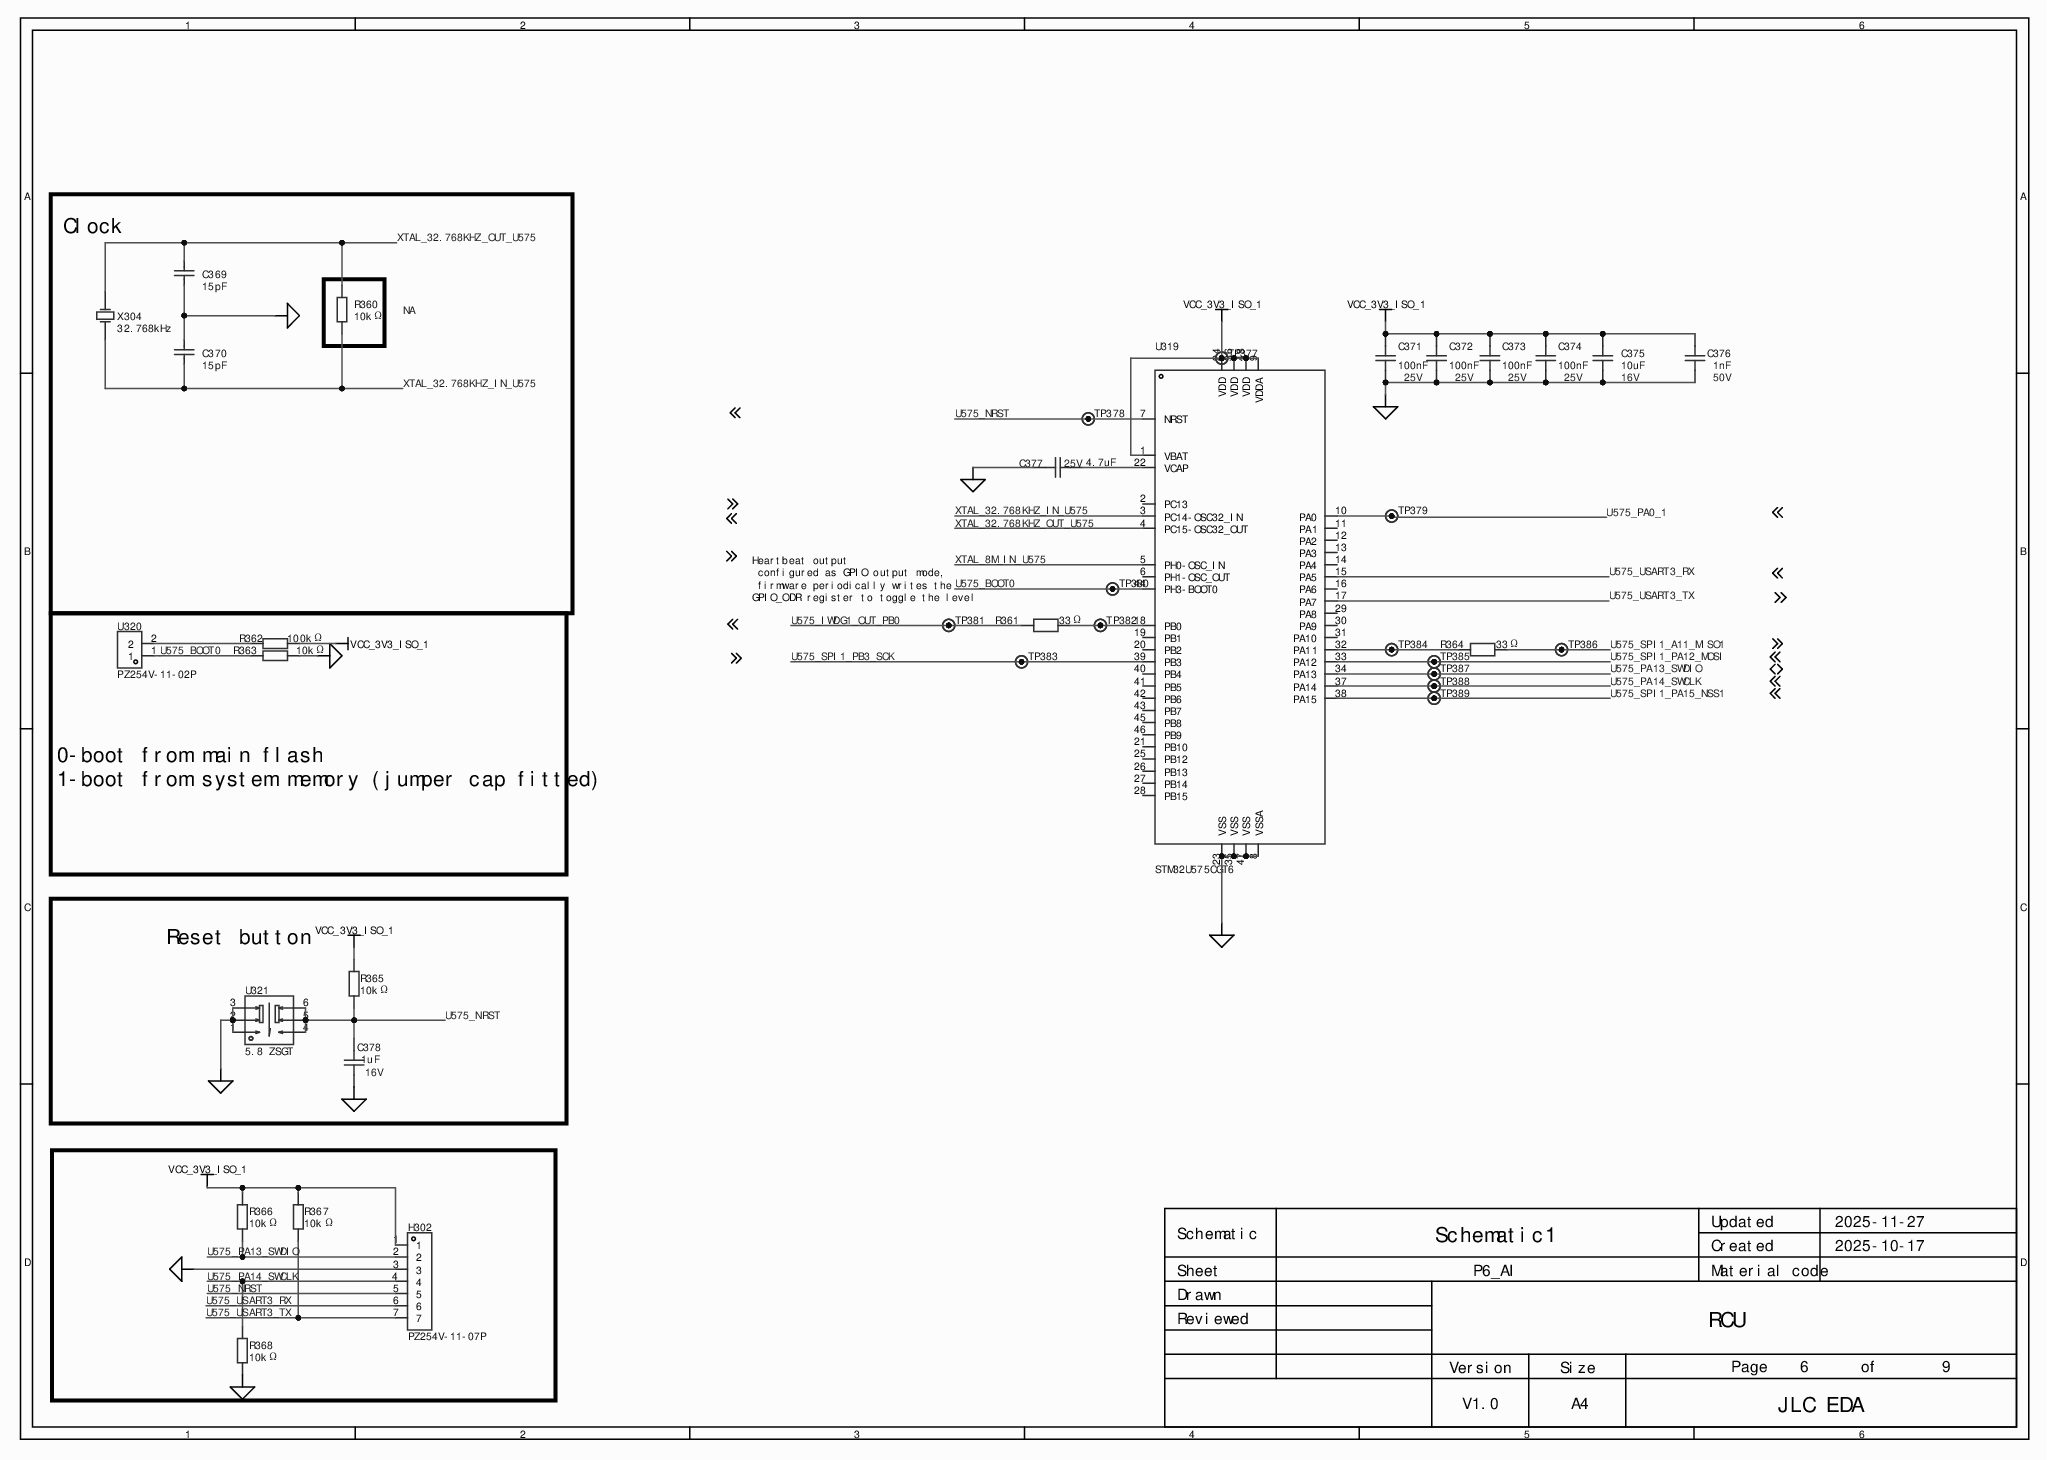
[diagram p0: MISC84429-7.SchDoc]
# Altium project MISC84429-12.PrjPcb (part 1 of 5)
9 sheets, 424 parts. Net scope: global (net labels, ports and power ports of the same name join across sheets).
Board file: MISC84429.PcbDoc
Sheets:
  MISC84429-7.SchDoc
  MISC84429-4.SchDoc
  MISC84429-3.SchDoc
  MISC84429-2.SchDoc
  MISC84429-5.SchDoc
  MISC84429-6.SchDoc
  MISC84429-8.SchDoc
  MISC84429-10.SchDoc
  MISC84429-9.SchDoc

## Sheet MISC84429-7.SchDoc
size 431 x 309 mm; Name: Sheet-Symbol; Symbol: Sheet-Symbol; Device: Sheet-Symbol

### Parts
C369  15pF  [C0402]
C370  15pF  [C0402]
C371  100nF  Voltage Rated: 25V  [C0603]
C372  100nF  Voltage Rated: 25V  [C0603]
C373  100nF  Voltage Rated: 25V  [C0603]
C374  100nF  Voltage Rated: 25V  [C0603]
C375  10uF  Voltage Rated: 16V  [C0805]
C376  1nF  Voltage Rated: 50V  [C0603]
C377  4.7uF  Voltage Rating: 25V  [C0603]
C378  1uF  Voltage Rated: 16V  [C0603]
H302  PZ254V-11-07P  [HDR-TH_7P-P2.54-V-M]
R360  10kΩ  [R0402]
R361  33Ω  [R0603]
R362  100kΩ  [R0603]
R363  10kΩ  [R0603]
R364  33Ω  [R0603]
R365  10kΩ  [R0603]
R366  10kΩ  [R0603]
R367  10kΩ  [R0603]
R368  10kΩ  [R0603]
TP377  (no value)  [Test-Point-0.5mm]
TP378  (no value)  [Test-Point-0.5mm]
TP379  (no value)  [Test-Point-0.5mm]
TP380  (no value)  [Test-Point-0.5mm]
TP381  (no value)  [Test-Point-0.5mm]
TP382  (no value)  [Test-Point-0.5mm]
TP383  (no value)  [Test-Point-0.5mm]
TP384  (no value)  [Test-Point-0.5mm]
TP385  (no value)  [Test-Point-0.5mm]
TP386  (no value)  [Test-Point-0.5mm]
TP387  (no value)  [Test-Point-0.5mm]
TP388  (no value)  [Test-Point-0.5mm]
TP389  (no value)  [Test-Point-0.5mm]
U319  STM32U575CGT6  [LQFP-48_L7.0-W7.0-P0.50-LS9.0-TL]
U320  PZ254V-11-02P  [HDR-TH_2P-P2.54-V-M]
U321  5.8 ZSGT  [SW-TH_5.8ZSGT]
X304  32.768kHz  [OSC-TH_BD3.1-P0.8-D0.3]

### Blocks framed on the sheet
Clock: C369 C370 R360 X304
Reset button: C378 R365 U321

### Nets
PGND: C369.1 C370.2 C371.2 C372.2 C373.2 C374.2 C375.1 C376.1 C377.2 C378.1 H302.3 R363.2 R368.2 U319.8(VSSA) U319.23(VSS) U319.35(VSS) U319.47(VSS) U321.1 U321.2 U321.3
VCC_3V3_ISO_1: C371.1 C372.1 C373.1 C374.1 C375.2 C376.2 H302.1 R362.2 R365.2 R366.2 R367.2 TP377.1 U319.1(VBAT) U319.9(VDDA) U319.24(VDD) U319.36(VDD) U319.48(VDD)
U575_BOOT0: R363.1 TP380.1 U319.44(PH3-BOOT0) U320.1
U575_IWDG1_OUT_PB0: R361.2 TP381.1
U575_NRST: C378.2 H302.5 R365.1 TP378.1 U319.7(NRST) U321.4 U321.5 U321.6
U575_PA0_1: TP379.1 U319.10(PA0)
U575_PA13_SWDIO: H302.2 R366.1 TP387.1 U319.34(PA13)
U575_PA14_SWCLK: H302.4 R368.1 TP388.1 U319.37(PA14)
U575_SPI1_A11_MISO1: R364.1 TP386.1
U575_SPI1_PA12_MOSI: TP385.1 U319.33(PA12)
U575_SPI1_PA15_NSS1: TP389.1 U319.38(PA15)
U575_SPI1_PB3_SCK: TP383.1 U319.39(PB3)
U575_USART3_RX: H302.6 U319.15(PA5)
U575_USART3_TX: H302.7 R367.1 U319.17(PA7)
XTAL_8M_IN_U575: U319.5(PH0-OSC_IN)
XTAL_32.768KHZ_IN_U575: C370.1 R360.1 U319.3(PC14-OSC32_IN) X304.1(OSC1)
XTAL_32.768KHZ_OUT_U575: C369.2 R360.2 U319.4(PC15-OSC32_OUT) X304.2(OSC2)
NetC377_1: C377.1 U319.22(VCAP)
NetR361_1: R361.1 TP382.1 U319.18(PB0)
NetR362_1: R362.1 U320.2
NetR364_2: R364.2 TP384.1 U319.32(PA11)

Not connected (* = marked no-connect by the designer): U319 2(PC13)* 6(PH1-OSC_OUT)* 11(PA1)* 12(PA2)* 13(PA3)* 14(PA4)* 16(PA6)* 19(PB1)* 20(PB2)* 21(PB10)* 25(PB12)* 26(PB13)* 27(PB14)* 28(PB15)* 29(PA8)* 30(PA9)* 31(PA10)* 40(PB4)* 41(PB5)* 42(PB6)* 43(PB7)* 45(PB8)* 46(PB9)*

### Notes on the sheet
- NA
- Heartbeat output
  configured as GPIO output mode,
  firmware periodically writes the
  GPIO_ODR register to toggle the level
- 0-boot from main flash
  1-boot from system memory (jumper cap fitted)
- 1
- 2
- 3
- 4
- 5
- 6
- A
- B
- C
- D
- Schematic
- Schematic1
- Created
- Updated
- 2025-11-27
- 2025-10-17
- Reviewed
- Drawn
- Sheet
- P6_AI
- Material code
- RCU
- Version
- Size
- Page
- of
- 9
- V1.0
- A4
- JLC EDA

### Library data of the parts
C369 C370 = GJM1555C1H150FB01D: Manufacturer: muRata(村田); Add into BOM: yes; Tolerance: ±1%; Voltage Rated: 50V; Temperature Coefficient: C0G; Symbol: GJM1555C1H150FB01D; Device: GJM1555C1H150FB01D; LCSC Part Name: 15pF ±1% 50V; Supplier Part: C441742; Manufacturer Part: GJM1555C1H150FB01D; Supplier Footprint: 0402; JLCPCB Part Class: Extended library; Datasheet: https://atta.szlcsc.com/upload/public/pdf/source/20200305/C490387_23319AE8C154DEB24C505E6C82A8106A.pdf; Supplier: LCSC; Convert to PCB: yes; Value: 15pF; Origin Footprint: C0402
C371-C374 = GRM188R71E104KA01D: Manufacturer: muRata(村田); Add into BOM: yes; Tolerance: ±10%; Temperature Coefficient: X7R; Symbol: GRM188R71E104KA01D; Device: GRM188R71E104KA01D; LCSC Part Name: 100nF ±10% 25V; Supplier Part: C77050; Manufacturer Part: GRM188R71E104KA01D; Supplier Footprint: 0603; JLCPCB Part Class: Extended library; Datasheet: https://atta.szlcsc.com/upload/public/pdf/source/20170622/1498103881034.pdf; Supplier: LCSC; Convert to PCB: yes; Value: 100nF; Origin Footprint: C0603
C375 = GRM21BR61C106KE15L: Manufacturer: muRata(村田); Add into BOM: yes; Tolerance: ±10%; Temperature Coefficient: X5R; Symbol: GRM21BR61C106KE15L; Device: GRM21BR61C106KE15L; LCSC Part Name: 10uF ±10% 16V; Supplier Part: C77075; Manufacturer Part: GRM21BR61C106KE15L; Supplier Footprint: 0805; JLCPCB Part Class: Extended library; Datasheet: https://atta.szlcsc.com/upload/public/pdf/source/20200305/C490387_23319AE8C154DEB24C505E6C82A8106A.pdf; Supplier: LCSC; Convert to PCB: yes; Value: 10uF; Origin Footprint: C0805
C376 = GRM1885C1H102JA01D: Manufacturer: muRata(村田); Add into BOM: yes; Tolerance: ±5%; Temperature Coefficient: C0G; Symbol: GRM1885C1H102JA01D; Device: GRM1885C1H102JA01D; LCSC Part Name: 1nF ±5% 50V; Supplier Part: C77026; Manufacturer Part: GRM1885C1H102JA01D; Supplier Footprint: 0603; JLCPCB Part Class: Extended library; Datasheet: https://atta.szlcsc.com/upload/public/pdf/source/20200305/C490387_23319AE8C154DEB24C505E6C82A8106A.pdf; Supplier: LCSC; Convert to PCB: yes; Value: 1nF; Origin Footprint: C0603
C377 = GRM188R61E475KE11D: Manufacturer: muRata(村田); Add into BOM: yes; Tolerance: ±10%; Temperature Coefficient: X5R; Symbol: GRM188R61E475KE11D; Device: GRM188R61E475KE11D; LCSC Part Name: 4.7uF ±10% 25V; Supplier Part: C90057; Manufacturer Part: GRM188R61E475KE11D; Supplier Footprint: 0603; JLCPCB Part Class: Extended library; Datasheet: https://item.szlcsc.com/datasheet/GRM188R61E475KE11D/91242.html; Supplier: LCSC; Convert to PCB: yes; Value: 4.7uF; Origin Footprint: C0603
C378 = GCM188R71C105KA64D: Manufacturer: muRata(村田); Add into BOM: yes; Tolerance: ±10%; Temperature Coefficient: X7R; Symbol: GCM188R71C105KA64D; Device: GCM188R71C105KA64D; LCSC Part Name: 1uF ±10% 16V; Supplier Part: C161212; Manufacturer Part: GCM188R71C105KA64D; Supplier Footprint: 0603; JLCPCB Part Class: Extended library; Datasheet: https://atta.szlcsc.com/upload/public/pdf/source/20181221/C161212_C96DD77354D5551432B3B7779E4D1948.pdf; Supplier: LCSC; Convert to PCB: yes; Value: 1uF; Origin Footprint: C0603
H302 = PZ254V-11-07P: Manufacturer: XFCN(兴飞); Add into BOM: yes; Pin Structure: 1x7P; Pitch: 2.54mm; Circluar Pins/Square Pins: Square pin; Symbol: PZ254V-11-07P; Device: PZ254V-11-07P; LCSC Part Name: 1x7P 间距:2.54mm 方针 直插; Supplier Part: C492406; Manufacturer Part: PZ254V-11-07P; Supplier Footprint: 插件,P=2.54mm; JLCPCB Part Class: Extended library; Datasheet: https://atta.szlcsc.com/upload/public/pdf/source/20200309/C492406_654C533EE691117E22DD9F76C114C2D9.pdf; Supplier: LCSC; Convert to PCB: yes; Row Spacing: -; Mounting Type: Through hole; Number of Rows: Single row; Number of Pins: 7P; Current Rating: -; Voltage Rating (Max): -; Length of Mating Pin: 6mm; Insulation Height: 2.5mm; Length of End Connection Pin: 3mm; Contact Material: Brass; Contact Plating: -; Operating Temperature: -40℃~+105℃; Color: Black; Origin Footprint: HDR-TH_7P-P2.54-V-M
R360 = 0402WGF1002TCE: Manufacturer: UNI-ROYAL(厚声); Add into BOM: yes; Tolerance: ±1%; Power(Watts): 62.5mW; Overload Voltage (Max): 50V; Temperature Coefficient: ±100ppm/℃; Symbol: 0402WGF1002TCE; Device: 0402WGF1002TCE; LCSC Part Name: 10kΩ ±1% 62.5mW 厚膜电阻; Supplier Part: C25744; Manufacturer Part: 0402WGF1002TCE; Supplier Footprint: 0402; JLCPCB Part Class: Basic library; Datasheet: https://atta.szlcsc.com/upload/public/pdf/source/20200306/C422600_1E6D84923E4A46A82E41ADD87F860B5C.pdf; Supplier: LCSC; Convert to PCB: yes; Type: Thick film resistor; Value: 10kΩ; Operating Temperature Range: -55℃~+155℃; Origin Footprint: R0402
R361 R364 = FRC0603F33R0TS: Manufacturer: FOJAN(富捷); Add into BOM: yes; Tolerance: ±1%; Power(Watts): 100mW; Voltage-Supply(Max): 75V; Temperature Coefficient: ±100ppm/℃; Symbol: FRC0603F33R0TS; Device: FRC0603F33R0TS; LCSC Part Name: 33Ω ±1% 100mW 厚膜电阻; Supplier Part: C2909394; Manufacturer Part: FRC0603F33R0TS; Supplier Footprint: 0603; JLCPCB Part Class: Extended library; Supplier: LCSC; Convert to PCB: yes; Type: Thick film resistor; Value: 33Ω; Operating Temperature: -55℃~+155℃; Origin Footprint: R0603
R362 = RC0603FR-07100KL: Manufacturer: YAGEO(国巨); Add into BOM: yes; Tolerance: ±1%; Power(Watts): 100mW; Overload Voltage (Max): 75V; Temperature Coefficient: ±100ppm/℃; Symbol: RC0603FR-07100KL; Device: RC0603FR-07100KL; LCSC Part Name: 厚膜电阻 100kΩ ±1% 100mW; Supplier Part: C14675; Manufacturer Part: RC0603FR-07100KL; Supplier Footprint: 0603; JLCPCB Part Class: Extended library; Datasheet: https://atta.szlcsc.com/upload/public/pdf/source/20140324/1457707028752.pdf; Supplier: LCSC; Convert to PCB: yes; Type: Thick film resistor; Value: 100kΩ; Operating Temperature Range: -55℃~+155℃; Origin Footprint: R0603
R363 R365-R368 = RC0603FR-0710KL: Manufacturer: YAGEO(国巨); Add into BOM: yes; Tolerance: ±1%; Power(Watts): 100mW; Overload Voltage (Max): 75V; Temperature Coefficient: ±100ppm/℃; Symbol: RC0603FR-0710KL; Device: RC0603FR-0710KL; LCSC Part Name: 厚膜电阻 10kΩ ±1% 100mW; Supplier Part: C98220; Manufacturer Part: RC0603FR-0710KL; Supplier Footprint: 0603; JLCPCB Part Class: Extended library; Datasheet: https://atta.szlcsc.com/upload/public/pdf/source/20180927/C295883_E8D83085EA81BD7DE0B2B681138C15EE.pdf; Supplier: LCSC; Convert to PCB: yes; Type: Thick film resistor; Value: 10kΩ; Operating Temperature Range: -55℃~+155℃; Origin Footprint: R0603
TP377-TP389 = Test-Point: Add into BOM: yes; Symbol: Test-Point; Device: Test-Point; Convert to PCB: yes; Origin Footprint: Test-Point-0.5mm
U319 = STM32U575CGT6: Manufacturer: ST(意法半导体); Add into BOM: yes; Symbol: STM32U575CGT6; Device: STM32U575CGT6; LCSC Part Name: 超低功耗带 FPU 的 Arm Cortex-M33 具有 Trust Zone，160 MHz MCU 带 1MB 闪存; Supplier Part: C5271006; Manufacturer Part: STM32U575CGT6; Supplier Footprint: LQFP-48(7x7); JLCPCB Part Class: Extended library; Datasheet: https://atta.szlcsc.com/upload/public/pdf/source/20250311/118E46867C2F8A0EF1AEA9206C957AC0.pdf; Supplier: LCSC; Convert to PCB: yes; Origin Footprint: LQFP-48_L7.0-W7.0-P0.50-LS9.0-TL
U320 = PZ254V-11-02P: Manufacturer: XFCN(兴飞); Add into BOM: yes; Pin Structure: 1x2P; Pitch: 2.54mm; Circluar Pins/Square Pins: Square pin; Symbol: PZ254V-11-02P; Device: PZ254V-11-02P; LCSC Part Name: 间距:2.54mm 1x2P 直插 方针; Supplier Part: C492401; Manufacturer Part: PZ254V-11-02P; Supplier Footprint: 插件,P=2.54mm; JLCPCB Part Class: Extended library; Datasheet: https://atta.szlcsc.com/upload/public/pdf/source/20200309/C492401_A812433581A9B211A7FFA413ADDFF0E5.pdf; Supplier: LCSC; Convert to PCB: yes; Row Spacing: -; Mounting Type: Through hole; Number of Rows: Single row; Number of Pins: 2P; Current Rating (Max): -; Voltage Rating (Max): -; Length of Mating Pin: 6mm; Insulation Height: 2.5mm; Length of End Connection Pin: 3mm; Contact Material: Brass; Contact Plating: -; Operating Temperature Range: -40℃~+105℃; Color: Black; Origin Footprint: HDR-TH_2P-P2.54-V-M
U321 = 5.8 ZSGT: Manufacturer: SHOU HAN(首韩); Add into BOM: yes; Circuit: DPDT; Self Lock / No Lock: Self-locking; Actuator Style: Square button; Contact Current: 110mA; Voltage Rating (DC): 30V; Insulation Resistance: 100MΩ; Actuator/Cap Color: White; With Lamp: Without; Pin Style: PC pin; Operating Force: 1.5N; Mechanical Life: 10 ten-thousand cycles; Symbol: 5.8 ZSGT; Device: 5.8 ZSGT; LCSC Part Name: 5.8*5.8有头/高头 带锁/自锁开关 泡泡机开关; Supplier Part: C2681587; Manufacturer Part: 5.8 ZSGT; Supplier Footprint: 插件; JLCPCB Part Class: Extended library; Datasheet: https://atta.szlcsc.com/upload/public/pdf/source/20210107/C2681587_CDDDDA4A1C7AC9FEB01815B75893A6BA.pdf; Supplier: LCSC; Convert to PCB: yes; Mounting Style: Through hole; Operating Temperature: -10℃~+70℃; Origin Footprint: SW-TH_5.8ZSGT
X304 = X308032768KGB2SC: Manufacturer: YXC(扬兴晶振); Add into BOM: yes; Normal temperature Frequency Tolerance: ±10ppm; Load Capacitance: 12.5pF; Frequency Stability: ±20ppm; Symbol: X308032768KGB2SC; Device: X308032768KGB2SC; LCSC Part Name: YT-38 32.768KHZ 2P 3080 12.5PF ±10PPM -20~70℃; Supplier Part: C52082; Manufacturer Part: X308032768KGB2SC; Supplier Footprint: DT-38; JLCPCB Part Class: Extended library; Datasheet: https://item.szlcsc.com/datasheet/X308032768KGB2SC/53096.html; Supplier: LCSC; Convert to PCB: yes; Type: Through-hole crystal; Value: 32.768kHz; Operating Temperature: -20℃~+70℃; Origin Footprint: OSC-TH_BD3.1-P0.8-D0.3

## Sheet MISC84429-4.SchDoc
size 431 x 309 mm; Name: Sheet-Symbol; Symbol: Sheet-Symbol; Device: Sheet-Symbol
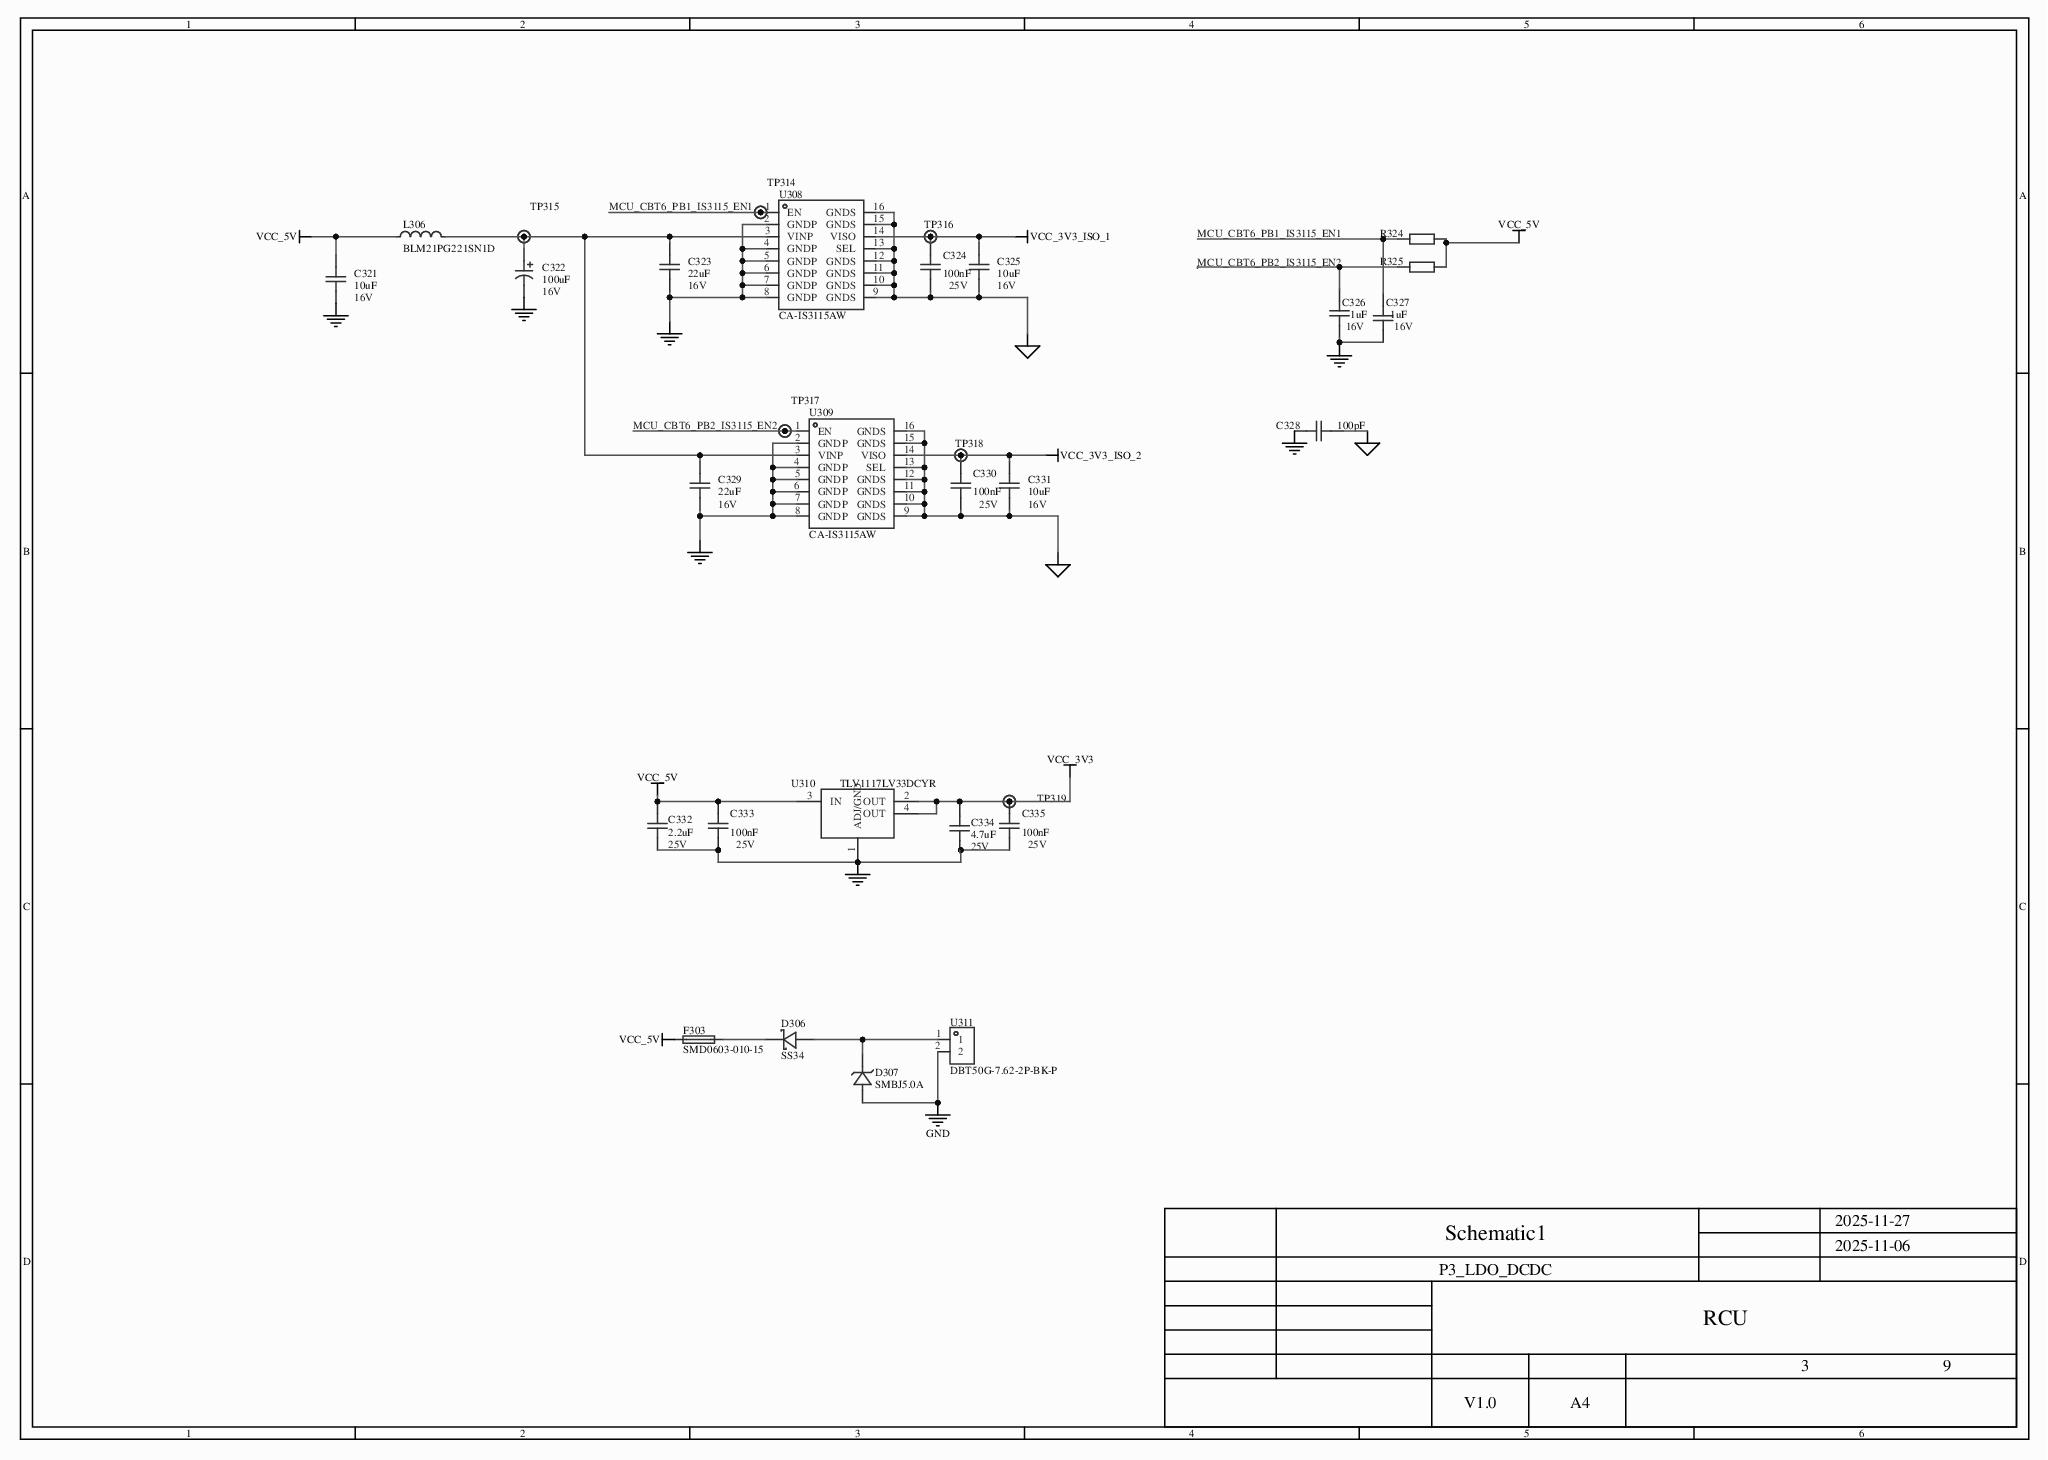
[diagram p1: MISC84429-4.SchDoc]

### Parts
C321  10uF  Voltage Rated: 16V  [C0805]
C322  100uF  Voltage Rating: 16V  [CAP-SMD_BD6.3-L6.6-W6.6-LS7.2-FD]
C323  22uF  Voltage Rating: 16V  [C0603]
C324  100nF  Voltage Rated: 25V  [C0603]
C325  10uF  Voltage Rated: 16V  [C0805]
C326  1uF  Voltage Rated: 16V  [C0603]
C327  1uF  Voltage Rated: 16V  [C0603]
C328  100pF  [CAP-TH_L7.0-W4.0-P10.00-D0.6]
C329  22uF  Voltage Rating: 16V  [C0603]
C330  100nF  Voltage Rated: 25V  [C0603]
C331  10uF  Voltage Rated: 16V  [C0805]
C332  2.2uF  Voltage Rating: 25V  [C0603]
C333  100nF  Voltage Rated: 25V  [C0603]
C334  4.7uF  Voltage Rating: 25V  [C0603]
C335  100nF  Voltage Rated: 25V  [C0603]
D306  SS34  [SMC_L6.9-W5.9-LS7.9-RD]
D307  SMBJ5.0A  [SMB_L4.6-W3.6-LS5.4-RD]
F303  SMD0603-010-15  [F0603]
L306  BLM21PG221SN1D  [L0805]
R324  (no value)  [R0603]
R325  (no value)  [R0603]
TP314  (no value)  [Test-Point-0.5mm]
TP315  (no value)  [Test-Point-0.5mm]
TP316  (no value)  [Test-Point-0.5mm]
TP317  (no value)  [Test-Point-0.5mm]
TP318  (no value)  [Test-Point-0.5mm]
TP319  (no value)  [Test-Point-0.5mm]
U308  CA-IS3115AW  [SOIC-16_L10.3-W7.5-P1.27-LS10.3-BL]
U309  CA-IS3115AW  [SOIC-16_L10.3-W7.5-P1.27-LS10.3-BL]
U310  TLV1117LV33DCYR  [SOT-223_L6.7-W3.5-P2.30-BR]
U311  DBT50G-7.62-2P-BK-P  [CONN-TH_2P-P7.62_L15.2-W16.7-EX4.2]

### Nets
GND: C321.1 C322.2 C323.1 C326.1 C327.1 C328.1 C329.1 C332.1 C333.2 C334.1 C335.2 D307.2(A) U308.2(GNDP) U308.4(GNDP) U308.5(GNDP) U308.6(GNDP) U308.7(GNDP) U308.8(GNDP) U309.2(GNDP) U309.4(GNDP) U309.5(GNDP) U309.6(GNDP) U309.7(GNDP) U309.8(GNDP) U310.1(ADJ/GND) U311.2
PGND: C324.2 C325.1 C328.2 C330.2 C331.1 U308.9(GNDS) U308.10(GNDS) U308.11(GNDS) U308.12(GNDS) U308.13(SEL) U308.15(GNDS) U308.16(GNDS) U309.9(GNDS) U309.10(GNDS) U309.11(GNDS) U309.12(GNDS) U309.13(SEL) U309.15(GNDS) U309.16(GNDS)
VCC_3V3: C334.2 C335.1 TP319.1 U310.2(OUT) U310.4(OUT)
VCC_3V3_ISO_1: C324.1 C325.2 TP316.1 U308.14(VISO)
VCC_3V3_ISO_2: C330.1 C331.2 TP318.1 U309.14(VISO)
VCC_5V: C321.2 C332.2 C333.1 F303.1 L306.1 R324.2 R325.2 U310.3(IN)
MCU_CBT6_PB1_IS3115_EN1: C327.2 R324.1 TP314.1 U308.1(EN)
MCU_CBT6_PB2_IS3115_EN2: C326.2 R325.1 TP317.1 U309.1(EN)
NetC322_1: C322.1 C323.2 C329.2 L306.2 TP315.1 U308.3(VINP) U309.3(VINP)
NetD306_1: D306.1(C) F303.2
NetD306_2: D306.2(A) D307.1(K) U311.1

### Notes on the sheet
- 1
- 2
- 3
- 4
- 5
- 6
- A
- B
- C
- D
- Schematic1
- 2025-11-27
- 2025-11-06
- P3_LDO_DCDC
- RCU
- 9
- V1.0
- A4

### Library data of the parts
C321 C325 C331 = GRM21BR61C106KE15L: Add into BOM: yes; Temperature Coefficient: X5R; Symbol: GRM21BR61C106KE15L; Device: GRM21BR61C106KE15L; Supplier Part: C77075; Manufacturer Part: GRM21BR61C106KE15L; Supplier Footprint: 0805; Datasheet: https://atta.szlcsc.com/upload/public/pdf/source/20200305/C490387_23319AE8C154DEB24C505E6C82A8106A.pdf; Supplier: LCSC; Convert to PCB: yes; Value: 10uF; Origin Footprint: C0805
C322 = RVT100UF16V67RV0016: Add into BOM: yes; Ripple Current: 93mA@120Hz; Symbol: RVT100UF16V67RV0016; Device: RVT100UF16V67RV0016; Supplier Part: C2887276; Manufacturer Part: RVT100UF16V67RV0016; Supplier Footprint: SMD,D6.3xL5.4mm; Datasheet: https://atta.szlcsc.com/upload/public/pdf/source/20240521/3810EB5B434F72326C196D6A9426C70A.pdf; Supplier: LCSC; Convert to PCB: yes; Value: 100uF; Equivalent Series Resistance(ESR): -; Diameter: 6.3mm; Height - Seated (Max): 5.4mm; Origin Footprint: CAP-SMD_BD6.3-L6.6-W6.6-LS7.2-FD
C323 C329 = GRM188R61C226ME01D: Add into BOM: yes; Temperature Coefficient: X5R; Symbol: GRM188R61C226ME01D; Device: GRM188R61C226ME01D; Supplier Part: C5116073; Manufacturer Part: GRM188R61C226ME01D; Supplier Footprint: 0603; Datasheet: https://item.szlcsc.com/datasheet/GRM188R61C226ME01D/5691201.html; Supplier: LCSC; Convert to PCB: yes; Value: 22uF; Origin Footprint: C0603
C324 C330 C333 C335 = GRM188R71E104KA01D: Add into BOM: yes; Temperature Coefficient: X7R; Symbol: GRM188R71E104KA01D; Device: GRM188R71E104KA01D; Supplier Part: C77050; Manufacturer Part: GRM188R71E104KA01D; Supplier Footprint: 0603; Datasheet: https://atta.szlcsc.com/upload/public/pdf/source/20170622/1498103881034.pdf; Supplier: LCSC; Convert to PCB: yes; Value: 100nF; Origin Footprint: C0603
C326 C327 = GCM188R71C105KA64D: Add into BOM: yes; Temperature Coefficient: X7R; Symbol: GCM188R71C105KA64D; Device: GCM188R71C105KA64D; Supplier Part: C161212; Manufacturer Part: GCM188R71C105KA64D; Supplier Footprint: 0603; Datasheet: https://atta.szlcsc.com/upload/public/pdf/source/20181221/C161212_C96DD77354D5551432B3B7779E4D1948.pdf; Supplier: LCSC; Convert to PCB: yes; Value: 1uF; Origin Footprint: C0603
C328 = Q07B1D101KN0B0N0N0: Add into BOM: yes; Voltage(AC): 500V; Ratings: Y1; Symbol: Q07B1D101KN0B0N0N0; Device: Q07B1D101KN0B0N0N0; Supplier Part: C22437611; Manufacturer Part: Q07B1D101KN0B0N0N0; Datasheet: https://item.szlcsc.com/datasheet/Q07B1D101KN0B0N0N0/24073310.html; Supplier: LCSC; Convert to PCB: yes; Value: 100pF; Origin Footprint: CAP-TH_L7.0-W4.0-P10.00-D0.6
C332 = GRM188R61E225KA12D: Add into BOM: yes; Temperature Coefficient: X5R; Symbol: GRM188R61E225KA12D; Device: GRM188R61E225KA12D; Supplier Part: C77047; Manufacturer Part: GRM188R61E225KA12D; Supplier Footprint: 0603; Datasheet: https://item.szlcsc.com/datasheet/GRM188R61E225KA12D/78174.html; Supplier: LCSC; Convert to PCB: yes; Value: 2.2uF; Origin Footprint: C0603
C334 = GRM188R61E475KE11D: Add into BOM: yes; Temperature Coefficient: X5R; Symbol: GRM188R61E475KE11D; Device: GRM188R61E475KE11D; Supplier Part: C90057; Manufacturer Part: GRM188R61E475KE11D; Supplier Footprint: 0603; Datasheet: https://item.szlcsc.com/datasheet/GRM188R61E475KE11D/91242.html; Supplier: LCSC; Convert to PCB: yes; Value: 4.7uF; Origin Footprint: C0603
D306 = SS34_C154551: Add into BOM: yes; Voltage - Forward(Vf@If): 500mV@3A; Voltage - DC Reverse(Vr): 40V; Current - Rectified: 3A; Reverse Leakage Current (Ir): 500uA@40V; Non-Repetitive Peak Forward Surge Current: 100A; Symbol: SS34_C154551; Device: SS34_C154551; Supplier Part: C154551; Manufacturer Part: SS34; Supplier Footprint: SMC(DO-214AB); Datasheet: https://item.szlcsc.com/datasheet/SS34/165893.html; Supplier: LCSC; Convert to PCB: yes; Origin Footprint: SMC_L6.9-W5.9-LS7.9-RD
D307 = SMBJ5.0A_C19077558: Add into BOM: yes; Reverse Stand-Off Voltage (Vrwm): 5V; Clamping Voltage: 9.2V; Peak Pulse Current (Ipp): 65.22A@10/1000us; Peak Pulse Power Dissipation (Ppp): 600W@10/1000us; Voltage - Breakdown: 7V; Reverse Leakage Current (Ir): 800uA; level of protection: IEC 61000-4-2; Type: TVS; Symbol: SMBJ5.0A_C19077558; Device: SMBJ5.0A_C19077558; Supplier Part: C19077558; Manufacturer Part: SMBJ5.0A; Supplier Footprint: DO-214AA(SMB); Datasheet: https://item.szlcsc.com/datasheet/SMBJ5.0A/20275643.html; Supplier: LCSC; Convert to PCB: yes; Origin Footprint: SMB_L4.6-W3.6-LS5.4-RD
F303 = SMD0603-010-15: Add into BOM: yes; Voltage - Max: 15V; Current - Max: 40A; Hold Current: 100mA; Trip Current: 300mA; Power Dissipation: 500mW; Time to Trip(Max): 600ms; Symbol: SMD0603-010-15; Device: SMD0603-010-15; LCSC Part Name: SMD0603-010-15; Supplier Part: C46640955; Manufacturer Part: SMD0603-010-15; Supplier Footprint: 0603; Datasheet: https://item.szlcsc.com/datasheet/SMD0603-010-15/48798661.html; Supplier: LCSC; Convert to PCB: yes; Length: 1.6mm; Width: 0.8mm; Origin Footprint: F0603
L306 = BLM21PG221SN1D: Add into BOM: yes; Current Rating: 2A; Circuits: 1; Symbol: BLM21PG221SN1D; Device: BLM21PG221SN1D; Supplier Part: C85840; Manufacturer Part: BLM21PG221SN1D; Supplier Footprint: 0805; Datasheet: https://atta.szlcsc.com/upload/public/pdf/source/20180326/C118443_3FAC30E9A4F0E6B81275543C61E0685E.pdf; Supplier: LCSC; Convert to PCB: yes; Origin Footprint: L0805
R324 R325 = RC0603FR-0710KL: Add into BOM: yes; Power(Watts): 100mW; Overload Voltage (Max): 75V; Symbol: RC0603FR-0710KL; Device: RC0603FR-0710KL; Supplier Part: C98220; Manufacturer Part: RC0603FR-0710KL; Supplier Footprint: 0603; Datasheet: https://atta.szlcsc.com/upload/public/pdf/source/20180927/C295883_E8D83085EA81BD7DE0B2B681138C15EE.pdf; Supplier: LCSC; Convert to PCB: yes; Origin Footprint: R0603